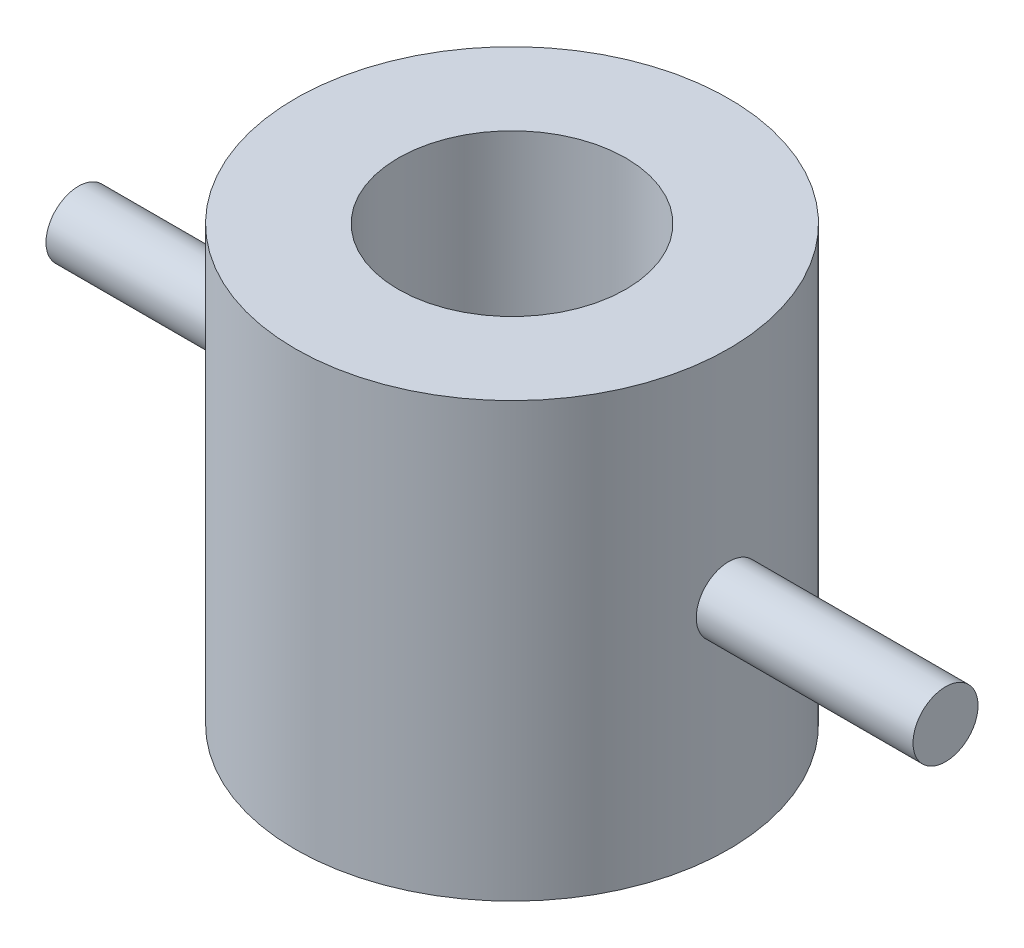
from build123d import *

# Parameters (mm, degrees)
SKETCH_2_R      = 20
SKETCH_2_R_2    = 10.5
EXTRUDE_1_DEPTH = 40
SKETCH_3_R      = 3
EXTRUDE_2_DEPTH = 20


with BuildPart() as part:
    # 草图2 → 凸台-拉伸1 (new body)
    with BuildSketch(Plane(origin=(0, 0, 0), x_dir=(1, 0, 0), z_dir=(0, 1, 0))):
        with Locations(Location((0, 0, 0), (0, 0, 270))):
            Circle(SKETCH_2_R)
        with Locations(Location((0, 0, 0), (0, 0, 270))):
            Circle(SKETCH_2_R_2, mode=Mode.SUBTRACT)
    extrude(amount=EXTRUDE_1_DEPTH)


with BuildPart() as body_2:
    # 草图3 → 凸台-拉伸2 (new body)
    with BuildSketch(Plane.ZY.offset(20)):
        with Locations((0, 20)):
            Circle(SKETCH_3_R)
    extrude(amount=EXTRUDE_2_DEPTH)


with BuildPart() as body_3:
    # 镜向3: mirrored copy
    add(body_2.part.mirror(Plane(origin=(0, 0, 0), x_dir=(0, 0, 1), z_dir=(1, 0, 0))))


solid = Compound([part.part, body_2.part, body_3.part])
